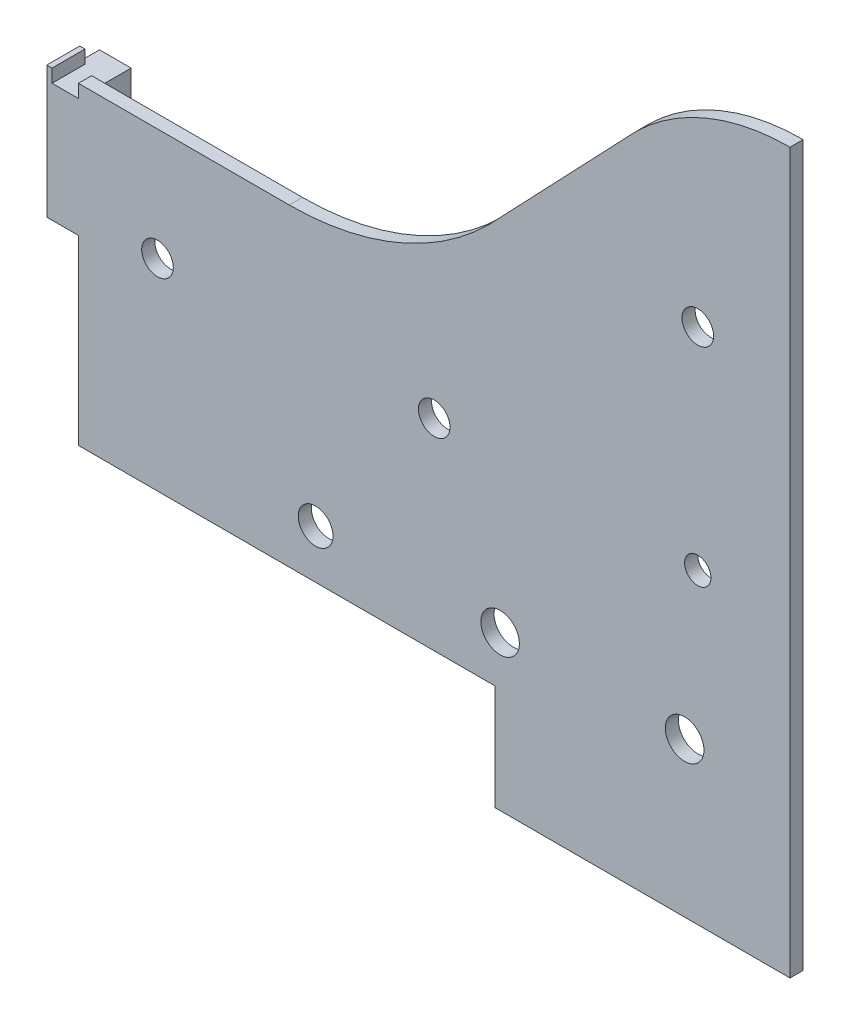
SolidWorks part; units mm, degrees
ref_plane "前视基准面" through (0, 0, 0) normal (0, 0, 1) x (1, 0, 0)
ref_plane "上视基准面" through (0, 0, 0) normal (0, 1, 0) x (1, 0, 0)
ref_plane "右视基准面" through (0, 0, 0) normal (1, 0, 0) x (0, 0, -1)
sketch "草图1" plane through (0, 0, 0) normal (0, 0, 1) x (1, 0, 0)
  line L6 (-86.7075, -188.9105) -> (103.2925, -188.9105)
  line L10 (-166.7075, -188.9105) -> (-86.7075, -188.9105)
  line L11 (-166.7075, -69.9105) -> (-86.7075, -69.9105)
  line L12 (-166.7075, -69.9105) -> (-166.7075, -188.9105)
  line L14 (103.2925, 44.0895) -> (103.2925, -188.9105)
  arc A6 (-86.7075, -69.9105) -> (-10.9437, -38.4674) centre (-86.7075, 37.0895) ccw
  arc A7 (103.2925, 44.0895) -> (44.6998, 19.8763) centre (103.2925, -38.9105) ccw
  spline S2 degree 2 poles (-10.9437, -38.4674) (16.8781, -9.2955) (44.6998, 19.8763) knots -0.00171 -0.00171 -0.00171 0.998178 0.998178 0.998178
extrude "凸台-拉伸3" add sketch "草图1" along normal blind 5 contours L11 A6 S2 A7 L14 L6 L10 L12
sketch "草图2" plane through (0, -69.9105, 0) normal (0, 1, 0) x (1, 0, 0)
  line L0 (-166.7075, -5) -> (-178.7075, -5)
  line L1 (-178.7075, -5) -> (-178.7075, 15)
  line L2 (-166.7075, -5) -> (-166.7075, 15)
  line L3 (-166.7075, 15) -> (-178.7075, 15)
  dimension "D1" = 12
  dimension "D2" = 20
extrude "凸台-拉伸4" add sketch "草图2" against normal blind 50
sketch "草图3" plane through (0, -69.9105, 0) normal (0, 1, 0) x (1, 0, 0)
  line L0 (-166.7075, 0) -> (-166.7075, -5)
  line L1 (-166.7075, -5) -> (-176.7202, -5)
  line L2 (-178.7075, -5) -> (-86.7075, -5) construction
  line L3 (-176.7202, -5) -> (-176.7202, 7.5)
  line L4 (-176.7202, 7.5) -> (-178.7075, 7.5)
  line L5 (-178.7075, 15) -> (-178.7075, -5) construction
  line L6 (-178.7075, 7.5) -> (-178.7075, 15)
  line L7 (-178.7075, 15) -> (-166.7075, 15)
  line L8 (-166.7075, 15) -> (-166.7075, 0)
extrude "切除-拉伸1" cut sketch "草图3" against normal blind 5
sketch "草图4" plane through (0, -188.9105, 0) normal (0, -1, 0) x (1, 0, 0)
  line L0 (-166.7075, 0) -> (103.2925, 0) construction
  line L1 (103.2925, 5) -> (-8.7075, 5)
  line L2 (103.2925, 5) -> (103.2925, 0)
  line L3 (103.2925, 0) -> (-8.7075, 0)
  line L4 (-8.7075, 5) -> (-8.7075, 0)
  dimension "D1" = 112
extrude "凸台-拉伸5" add sketch "草图4" along normal blind 40
extrude "切除-拉伸2" cut sketch "草图5" against normal up to surface (25 mm away)
sketch "草图5" plane through (703.4188, 634.2319, 5) normal (0, 0, 1) x (0, 1, 0)
  circle A0 centre (-666.7043, 635.1263) radius 6
  circle A1 centre (-746.7043, 635.1263) radius 5
  circle A2 centre (-746.7043, 840.1263) radius 6
  circle A3 centre (-746.7043, 735.1263) radius 6
extrude "切除-拉伸3" cut sketch "草图6" against normal up to surface (45 mm away)
sketch "草图6" plane through (703.4188, 634.2319, 15) normal (0, 0, 1) x (0, 1, 0)
  circle A0 centre (-804.6425, 640.1263) radius 7.3329
  circle A1 centre (-804.6425, 710.1263) radius 7.3013
  circle A2 centre (-804.6425, 780.1263) radius 6.6032
